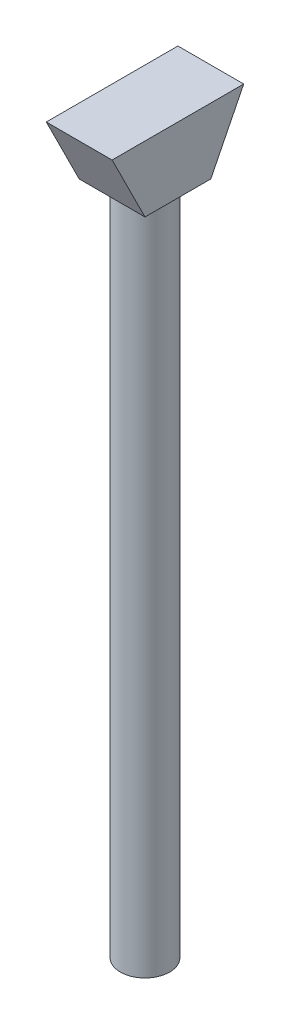
SolidWorks part; units mm, degrees
material "Q235-A"
ref_plane "Front Plane" through (0, 0, 0) normal (0, 0, 1) x (1, 0, 0)
ref_plane "Top Plane" through (0, 0, 0) normal (0, 1, 0) x (1, 0, 0)
ref_plane "Right Plane" through (0, 0, 0) normal (1, 0, 0) x (0, 0, -1)
sketch "Sketch1" plane through (0, 0, 0) normal (1, 0, 0) x (0, 0, -1)
  line L1 (40, -20) -> (-40, -20)
  line L2 (40, -20) -> (40, 20)
  line L3 (40, 20) -> (-40, 20)
  line L4 (-40, -20) -> (-40, 20)
  line L5 (40, -20) -> (-40, 20) construction
  line L6 (40, 20) -> (-40, -20) construction
  point P0 (0, 0)
  dimension "D1" = 80
  dimension "D2" = 40
extrude "Boss-Extrude1" add sketch "Sketch1" along normal mid plane 40
sketch "Sketch2" plane through (0, 0, 0) normal (1, 0, 0) x (0, 0, -1)
  line L0 (-40, 20) -> (-20, -20)
  line L1 (-40, -20) -> (40, -20) construction
  line L2 (-20, -20) -> (-40, -20)
  line L3 (-40, -20) -> (-40, 20)
  line L4 (0, 0) -> (0, -32.9014) construction
  line L5 (40, 20) -> (40, -20)
  line L6 (40, -20) -> (20, -20)
  line L7 (20, -20) -> (40, 20)
  dimension "D1" = 40
extrude "Cut-Extrude1" cut sketch "Sketch2" against normal through all both and the other way through all
sketch "Sketch3" plane through (0, -20, 0) normal (0, -1, 0) x (1, 0, 0)
  circle A0 centre (0, 0) radius 15
  dimension "D1" = 30
extrude "Boss-Extrude2" add sketch "Sketch3" along normal blind 410
